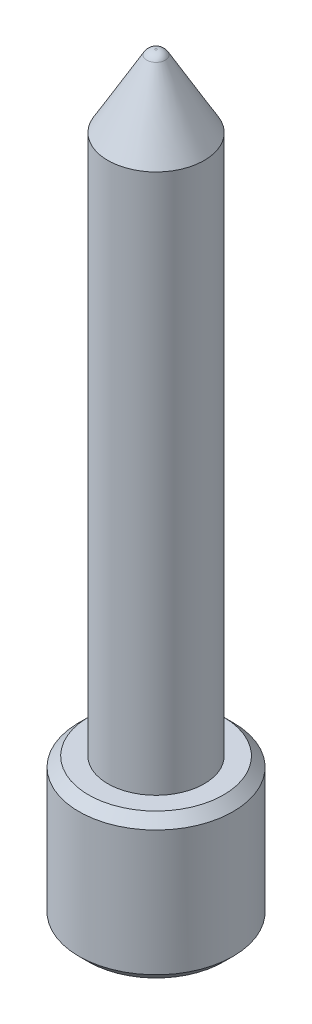
SolidWorks part; units mm, degrees
ref_plane "Front Plane" through (0, 0, 0) normal (0, 0, 1) x (1, 0, 0)
ref_plane "Top Plane" through (0, 0, 0) normal (0, 1, 0) x (1, 0, 0)
ref_plane "Right Plane" through (0, 0, 0) normal (1, 0, 0) x (0, 0, -1)
other "Configuration Table"
sketch "Sketch1" plane through (0, 0, 0) normal (0, 0, 1) x (1, 0, 0)
  line L0 (0, 0) -> (0, 78.4916) construction
  line L1 (-0.9634, 77.9916) -> (-5, 71)
  line L2 (-5, 71) -> (-5, 15)
  line L3 (-5, 15) -> (-8, 15)
  line L4 (-8, 15) -> (-8, 0)
  line L5 (-8, 0) -> (0, 0)
  line L6 (0, 0) -> (0, 78.4916)
  line L7 (-0.0974, 78.4916) -> (0, 78.4916)
  arc A0 (-0.0974, 78.4916) -> (-0.9634, 77.9916) centre (-0.0974, 77.4916) ccw
  dimension "D6" = 1
  dimension "D1" = 5
  dimension "D2" = 8
  dimension "D3" = 15
  dimension "D4" = 56
  dimension "D5" = 30
revolve "Revolve1" add sketch "Sketch1" angle 360 about L0
chamfer "Chamfer1" distance 1 angle 45 2 edges at (0, 15, -8) (0, 0, -8)
